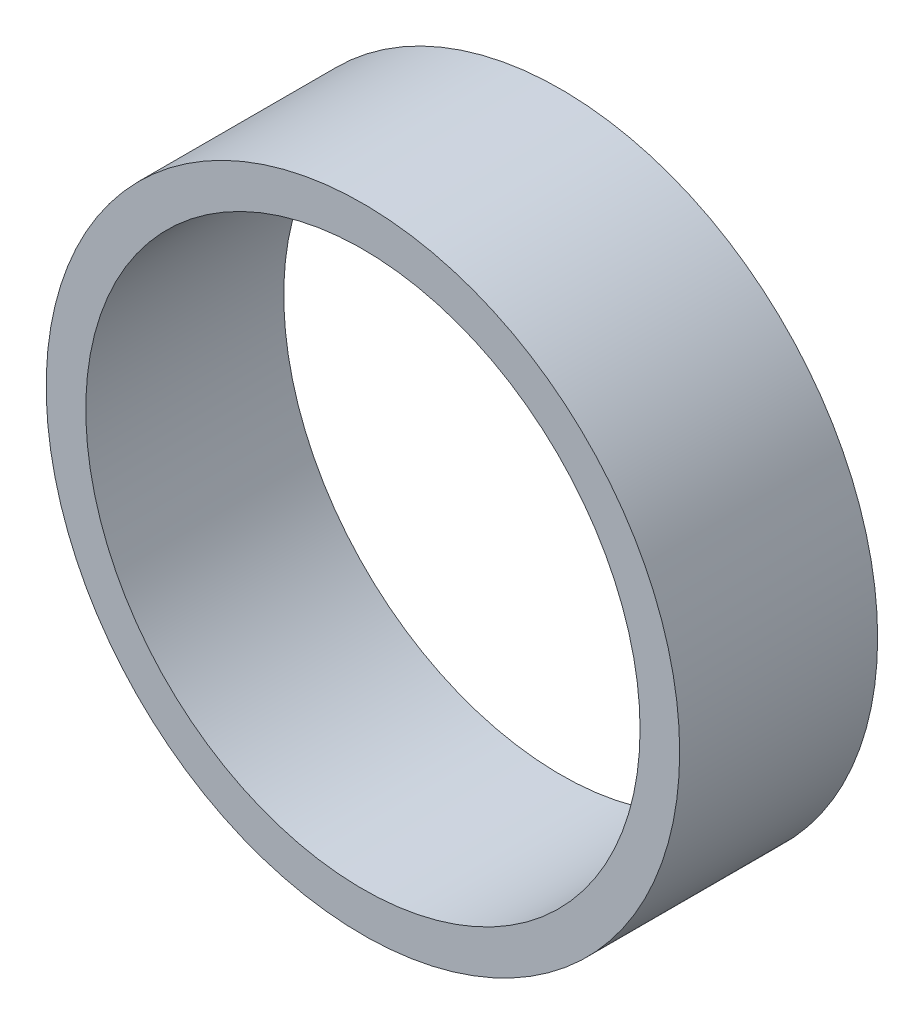
from build123d import *

# Parameters (mm, degrees)
SKETCH_1_R      = 40
SKETCH_1_R_2    = 35
EXTRUDE_1_DEPTH = 12.5


with BuildPart() as part:
    # 草图1 → 凸台-拉伸1 (new, symmetric)
    with BuildSketch(Plane.XY):
        Circle(SKETCH_1_R)
        Circle(SKETCH_1_R_2, mode=Mode.SUBTRACT)
    extrude(amount=EXTRUDE_1_DEPTH, both=True)


solid = part.part
